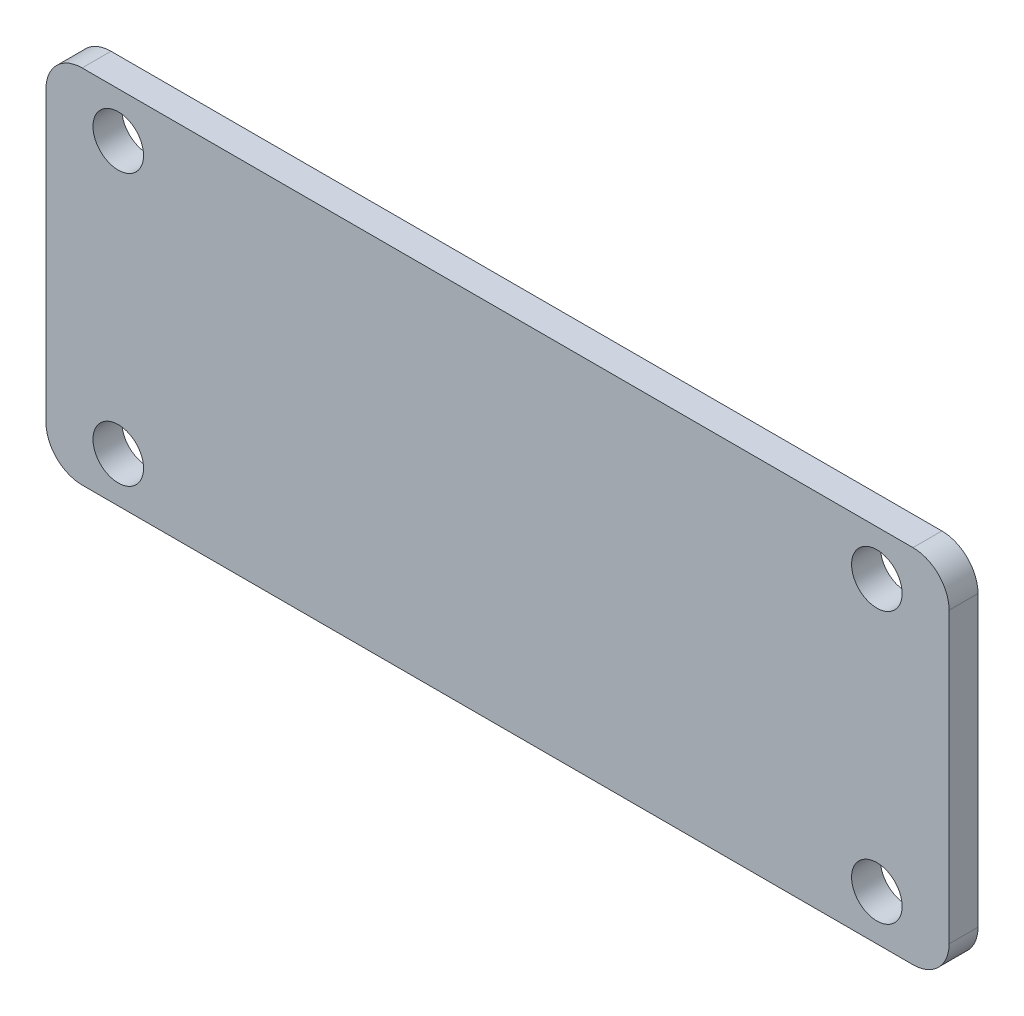
SolidWorks part; units mm, degrees
material "Q235B"
ref_plane "Front Plane" through (0, 0, 0) normal (0, 0, 1) x (1, 0, 0)
ref_plane "Top Plane" through (0, 0, 0) normal (0, 1, 0) x (1, 0, 0)
ref_plane "Right Plane" through (0, 0, 0) normal (1, 0, 0) x (0, 0, -1)
sketch "Sketch1" plane through (0, 0, 0) normal (0, 0, 1) x (1, 0, 0)
  line L1 (125, -50) -> (-125, -50)
  line L2 (125, -50) -> (125, 50)
  line L3 (125, 50) -> (-125, 50)
  line L4 (-125, -50) -> (-125, 50)
  line L5 (125, -50) -> (-125, 50) construction
  line L6 (125, 50) -> (-125, -50) construction
  point P0 (0, 0)
  dimension "D1" = 100
  dimension "D2" = 250
extrude "Boss-Extrude1" add sketch "Sketch1" along normal mid plane 8
hole_wizard "Ø14.0 (14) Diameter Hole1" positions "Sketch2" profile "Sketch3" hole size "Ø14.0" standard "GB" end condition up to next
sketch "Sketch2" plane through (0, 0, 4) normal (0, 0, 1) x (1, 0, 0)
  line L0 (0, 50) -> (0, 0) construction
  line L1 (125, 50) -> (-125, 50) construction
  line L2 (0, 0) -> (-125, 0) construction
  line L3 (-125, 50) -> (-125, -50) construction
  point P0 (-105, 37.5)
  point P13 (105, 37.5)
  point P14 (105, -37.5)
  point P15 (-105, -37.5)
  dimension "D1" = 210
  dimension "D2" = 75
sketch "Sketch3" plane through (-105, 37.5, 4) normal (1, 0, 0) x (0, -1, 0)
  line L0 (0, 0) -> (0, 8)
  line L1 (0, 8) -> (7, 8)
  line L2 (7, 8) -> (7, 0)
  line L5 (7, 0) -> (0, 0)
  line L11 (0, -6.35) -> (0, 107.95) construction
  dimension "通孔孔直径" = 14
  dimension "通孔孔深度" = 8
chamfer "Chamfer1" [suppressed] distance 10 angle 45
fillet "Fillet1" radius 10 4 edges at (125, 50, 0) (125, -50, 0) (-125, -50, 0) (-125, 50, 0)
